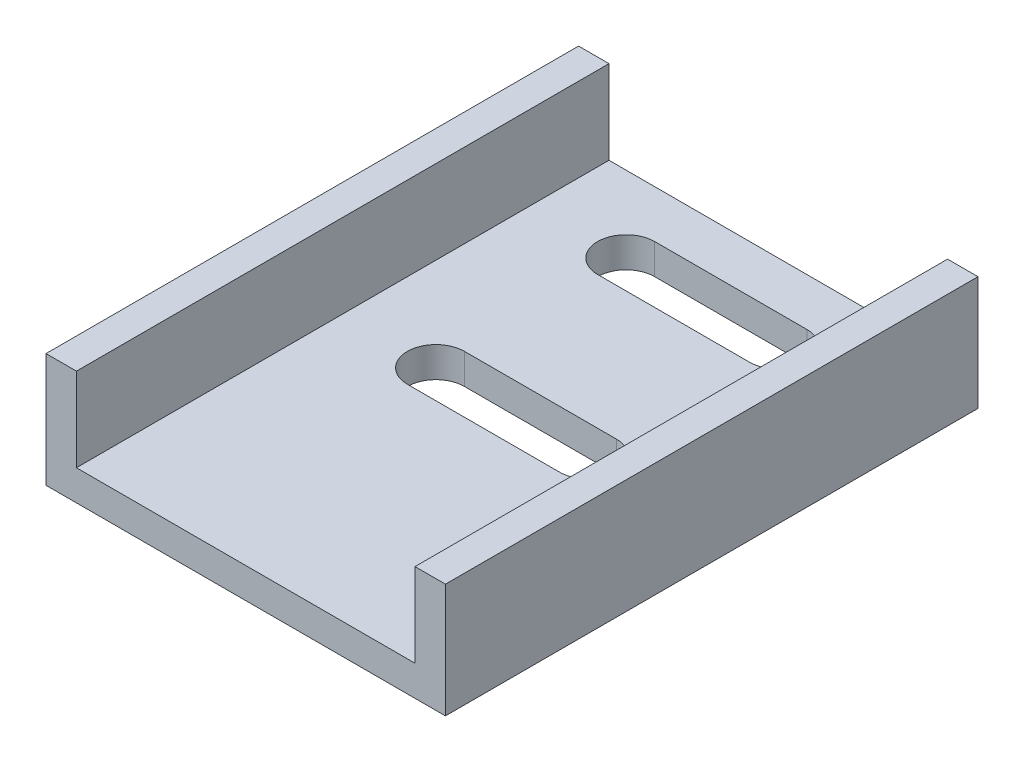
SolidWorks part; units mm, degrees
ref_plane "前视基准面" through (0, 0, 0) normal (0, 0, 1) x (1, 0, 0)
ref_plane "上视基准面" through (0, 0, 0) normal (0, 1, 0) x (1, 0, 0)
ref_plane "右视基准面" through (0, 0, 0) normal (1, 0, 0) x (0, 0, -1)
sketch "草图1" plane through (0, 0, 0) normal (0, 0, 1) x (1, 0, 0)
  line L0 (0, 0) -> (105, 0)
  line L1 (105, 0) -> (105, 30)
  line L2 (0, 0) -> (0, 30)
  line L3 (8, 8) -> (8, 30)
  line L4 (8, 8) -> (97, 8)
  line L5 (97, 8) -> (97, 30)
  line L6 (0, 30) -> (8, 30)
  line L7 (97, 30) -> (105, 30)
  dimension "D1" = 8
extrude "凸台-拉伸1" add sketch "草图1" along normal blind 140
sketch "草图2" plane through (0, 0, 0) normal (0, -1, 0) x (1, 0, 0)
  line L4 (0, 0) -> (105, 0)
  line L6 (52.5, 0) -> (52.5, 20)
  line L7 (52.5, 27.5) -> (52.5, 12.5)
  line L8 (32.5, 12.5) -> (72.5, 12.5)
  line L9 (32.5, 27.5) -> (72.5, 27.5)
  line L10 (52.5, 20) -> (52.5, 70)
  line L11 (32.5, 77.5) -> (72.5, 77.5)
  line L12 (52.5, 77.5) -> (52.5, 62.5)
  line L13 (32.5, 62.5) -> (72.5, 62.5)
  arc A2 (72.5, 12.5) -> (72.5, 27.5) centre (72.5, 20) ccw
  arc A3 (32.5, 27.5) -> (32.5, 12.5) centre (32.5, 20) ccw
  arc A4 (32.5, 77.5) -> (32.5, 62.5) centre (32.5, 70) ccw
  arc A5 (72.5, 62.5) -> (72.5, 77.5) centre (72.5, 70) ccw
extrude "切除-拉伸1" cut sketch "草图2" against normal blind 140 contours L13 A5 L11 L12 L10 | L11 A4 L13 L10 L12 | L9 A3 L8 L6 L7 | L8 A2 L9 L7 L6
